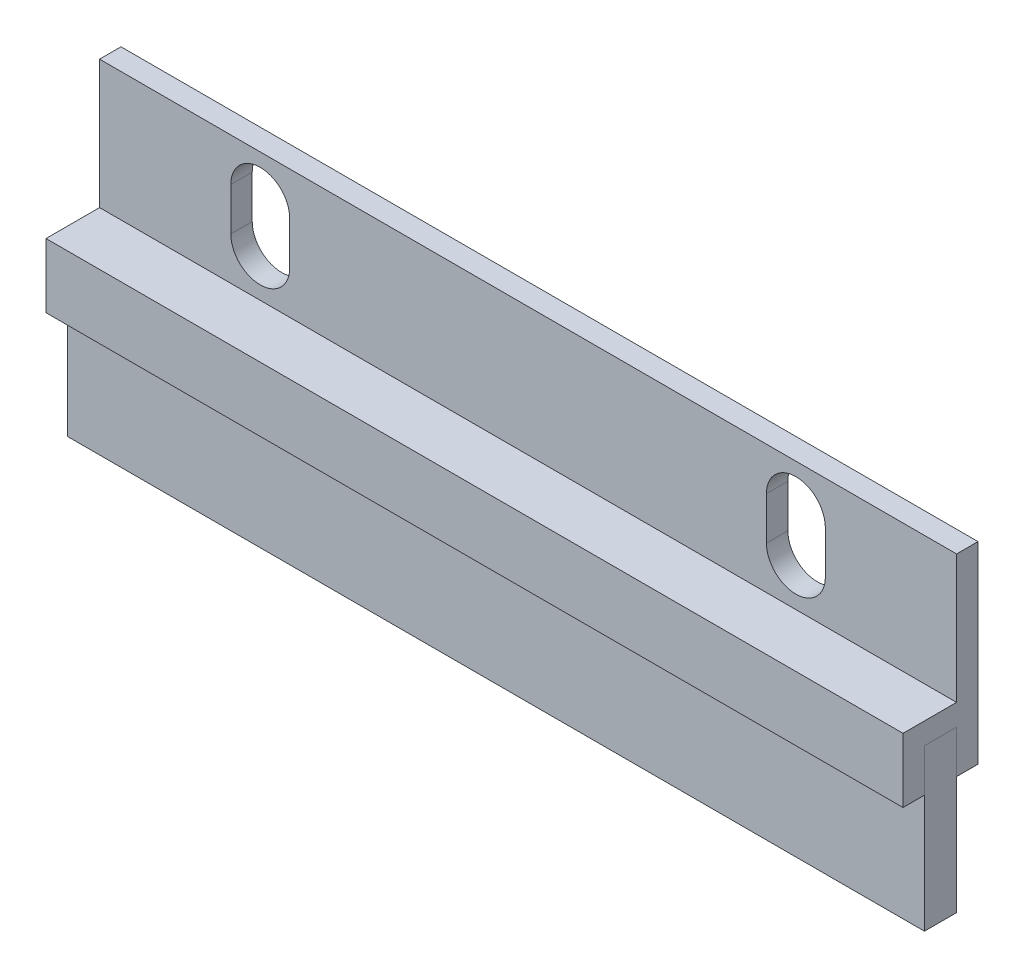
from build123d import *

# Parameters (mm, degrees)
SKETCH_1_W          = 80
SKETCH_1_H          = 18
EXTRUDE_1_DEPTH     = 2
SKETCH_2_W          = 80
SKETCH_2_H          = 2
EXTRUDE_2_DEPTH     = 3
SKETCH_3_W          = 80
SKETCH_3_H          = 2
EXTRUDE_3_DEPTH     = 6
SKETCH_5_W          = 80
SKETCH_5_H          = 3
EXTRUDE_5_DEPTH     = 15
CUT_EXTRUDE_1_DEPTH = 5


with BuildPart() as part:
    # 草图1 → 凸台-拉伸1 (new body)
    with BuildSketch(Plane.XY):
        with Locations((0, 9)):
            Rectangle(SKETCH_1_W, SKETCH_1_H)
    extrude(amount=EXTRUDE_1_DEPTH)

    # 草图2 → 凸台-拉伸2 (add)
    with BuildSketch(Plane.XY.offset(2)):
        with Locations((0, 5)):
            Rectangle(SKETCH_2_W, SKETCH_2_H)
    extrude(amount=EXTRUDE_2_DEPTH)

    # 草图3 → 凸台-拉伸3 (add)
    with BuildSketch(Plane(origin=(0, 6, 0), x_dir=(1, 0, 0), z_dir=(0, 1, 0))):
        with Locations((0, -6)):
            Rectangle(SKETCH_3_W, SKETCH_3_H)
    extrude(amount=-EXTRUDE_3_DEPTH)

    # 草图6 → 切除-拉伸1 (cut)
    with BuildSketch(Plane.XY.offset(2)):
        with BuildLine():
            Line((-22.25, 14), (-22.25, 10))
            ThreePointArc((-22.25, 10), (-25, 7.25), (-27.75, 10))
            Line((-27.75, 10), (-27.75, 14))
            ThreePointArc((-27.75, 14), (-25, 16.75), (-22.25, 14))
        make_face()
    cut_extrude_1 = extrude(amount=-CUT_EXTRUDE_1_DEPTH, mode=Mode.SUBTRACT)

    # 镜向1: 切除-拉伸1 across plane
    add(cut_extrude_1.mirror(Plane.ZY), mode=Mode.SUBTRACT)


with BuildPart() as body_2:
    # 草图5 → 凸台-拉伸5 (new body)
    with BuildSketch(Plane.XZ.offset(-4)):
        with Locations((0, 3.5)):
            Rectangle(SKETCH_5_W, SKETCH_5_H)
    extrude(amount=EXTRUDE_5_DEPTH)


solid = Compound([part.part, body_2.part])
